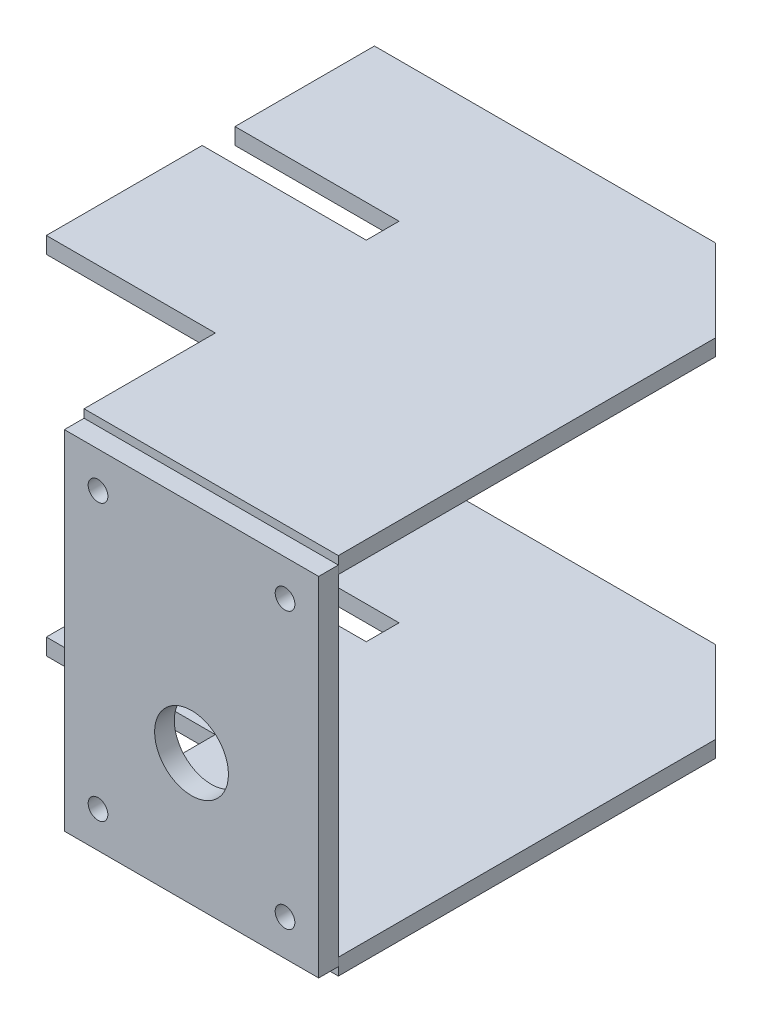
from build123d import *

# Parameters (mm, degrees)
SKETCH1_W                  = 155
SKETCH1_H                  = 212
BOSS_EXTRUDE1_DEPTH        = 12
F_12_0_12_DIAMETER_HOLE1_D = 12
BOSS_EXTRUDE2_DEPTH        = 5
CHAMFER1_SIZE              = 50
SKETCH9_R                  = 22.5
CUT_EXTRUDE2_DEPTH         = 12
SKETCH10_W                 = 100
SKETCH10_H                 = 20
CUT_EXTRUDE3_DEPTH         = 401.33017623


with BuildPart() as part:
    # Sketch1 → Boss-Extrude1 (new body)
    with BuildSketch(Plane.XY):
        Rectangle(SKETCH1_W, SKETCH1_H)
    extrude(amount=BOSS_EXTRUDE1_DEPTH)

    # Ø12.0 (12) Diameter Hole1 (through all)
    with Locations(Plane(origin=(0, 0, 0), x_dir=(-1, 0, 0), z_dir=(0, 0, -1))):
        with Locations((-57, 84), (57, 84), (-57, -84), (57, -84)):
            Hole(F_12_0_12_DIAMETER_HOLE1_D / 2)

    # Sketch9 → Cut-Extrude2 (cut)
    with BuildSketch(Plane(origin=(0, 0, 0), x_dir=(-1, 0, 0), z_dir=(0, 0, -1))):
        with Locations((0, -26)):
            Circle(SKETCH9_R)
    extrude(amount=-CUT_EXTRUDE2_DEPTH, mode=Mode.SUBTRACT)


with BuildPart() as body_2:
    # Sketch8 → Boss-Extrude2 (new, symmetric)
    with BuildSketch(Plane(origin=(0, 106, 0), x_dir=(1, 0, 0), z_dir=(0, 1, 0))):
        Polygon((77.5, 0), (-77.5, 0), (-77.5, 80), (-180.5, 80), (-180.5, 280), (77.5, 280), align=None)
    extrude(amount=BOSS_EXTRUDE2_DEPTH, both=True)

    # Chamfer1
    chamfer1_edges = [body_2.edges().sort_by_distance(p)[0] for p in [
        (77.5, 106, -280),
    ]]
    chamfer(chamfer1_edges, length=CHAMFER1_SIZE)


with BuildPart() as body_3:
    # Mirror1: mirrored copy
    add(body_2.part.mirror(Plane.ZX))


with BuildPart() as cut_extrude3_tool:
    # Sketch10 → Cut-Extrude3 (new, through all)
    with BuildSketch(Plane(origin=(0, 111, 0), x_dir=(1, 0, 0), z_dir=(0, 1, 0))):
        with Locations((-130.5, 185)):
            Rectangle(SKETCH10_W, SKETCH10_H)
    extrude(amount=-CUT_EXTRUDE3_DEPTH)


with BuildPart() as body_2_1:
    add(body_2.part)

    # Cut-Extrude3: cut by cut_extrude3_tool
    add(cut_extrude3_tool.part, mode=Mode.SUBTRACT)


with BuildPart() as body_3_1:
    add(body_3.part)

    # Cut-Extrude3: cut by cut_extrude3_tool
    add(cut_extrude3_tool.part, mode=Mode.SUBTRACT)


solid = Compound([part.part, body_2_1.part, body_3_1.part])
